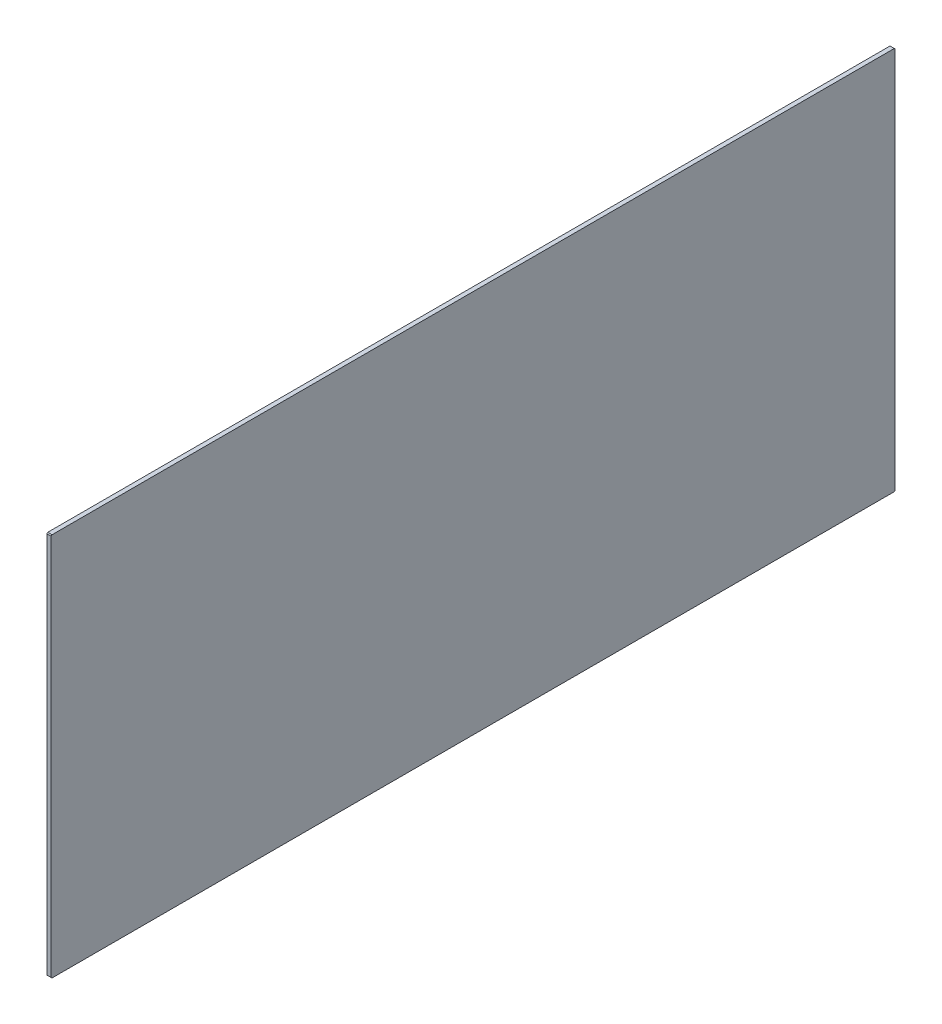
from build123d import *

# Parameters (mm, degrees)
SKETCH_2_W      = 985
SKETCH_2_H      = 448
EXTRUDE_1_DEPTH = 5
CHAMFER_1_SIZE  = 1


with BuildPart() as part:
    # 草图2 → 凸台-拉伸1 (new body)
    with BuildSketch(Plane(origin=(0, 0, 0), x_dir=(0, 0, -1), z_dir=(1, 0, 0))):
        Rectangle(SKETCH_2_W, SKETCH_2_H)
    extrude(amount=EXTRUDE_1_DEPTH)

    # 倒角1
    chamfer_1_edges = [part.edges().sort_by_distance(p)[0] for p in [
        (2.5, -224, -492.5),
        (2.5, -224, 492.5),
        (2.5, 224, 492.5),
        (2.5, 224, -492.5),
    ]]
    chamfer(chamfer_1_edges, length=CHAMFER_1_SIZE)


solid = part.part
